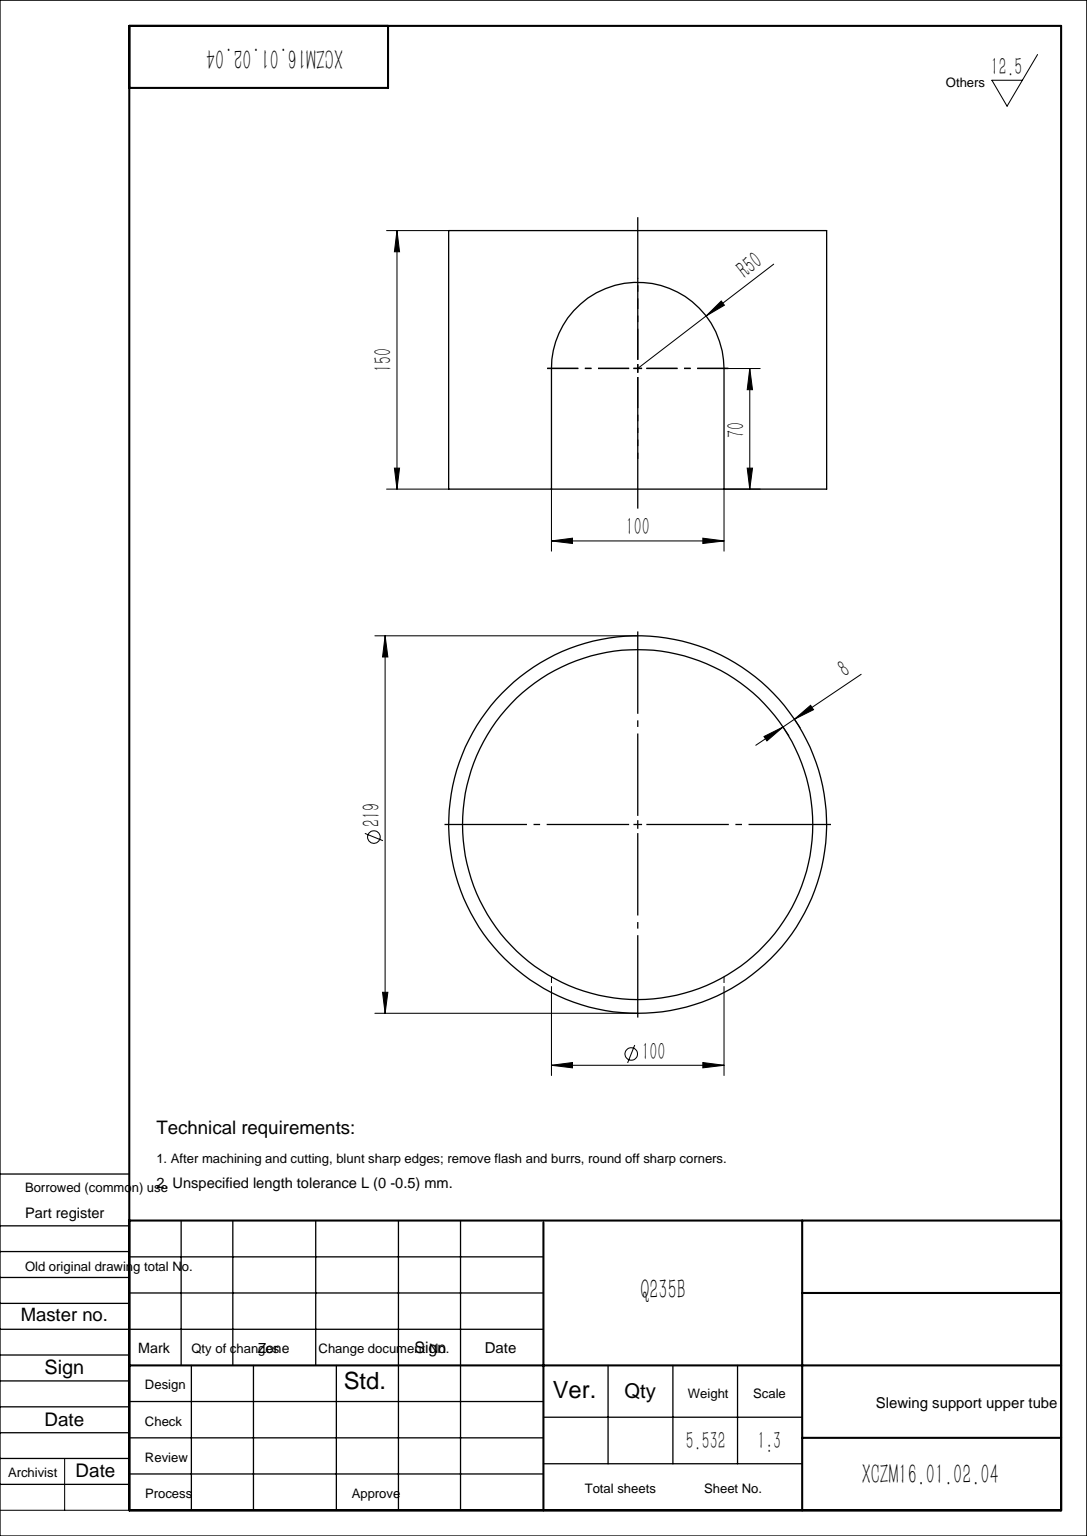
from build123d import *

# Parameters (mm, degrees)
SKETCH1_R               = 109.5
SKETCH1_R_2             = 101.5
BOSS_EXTRUDE1_DEPTH     = 150
CUT_EXTRUDE1_REACH      = 217.593
CUT_EXTRUDE1_END_RADIUS = 109.5


with BuildPart() as part:
    # Sketch1 → Boss-Extrude1 (new body)
    with BuildSketch(Plane(origin=(0, 0, 0), x_dir=(1, 0, 0), z_dir=(0, 1, 0))):
        with Locations(Location((0, 0, 0), (0, 0, 270))):
            Circle(SKETCH1_R)
        with Locations(Location((0, 0, 0), (0, 0, 270))):
            Circle(SKETCH1_R_2, mode=Mode.SUBTRACT)
    extrude(amount=BOSS_EXTRUDE1_DEPTH)

    # Cut-Extrude1: up to this cylinder (the profile starts inside it)
    cut_extrude1_end = Plane(origin=(0, 35, 0), z_dir=(0, -1, 0)) * Cylinder(CUT_EXTRUDE1_END_RADIUS, 655.186, mode=Mode.PRIVATE)
    # Sketch2 → Cut-Extrude1 (cut, up to the surface)
    with BuildSketch(Plane.XY, mode=Mode.PRIVATE) as cut_extrude1_sk1:
        with BuildLine():
            Line((-50, 0), (-50, 70))
            ThreePointArc((-50, 70), (0, 120), (50, 70))
            Line((50, 70), (50, 0))
            ThreePointArc((50, 0), (0, -50), (-50, 0))
        make_face()
    cut_extrude1_tool1 = extrude(cut_extrude1_sk1.sketch, amount=CUT_EXTRUDE1_REACH, mode=Mode.PRIVATE) & cut_extrude1_end
    add(cut_extrude1_tool1.solids().sort_by_distance((0, 35, 0))[0], mode=Mode.SUBTRACT)


solid = part.part
